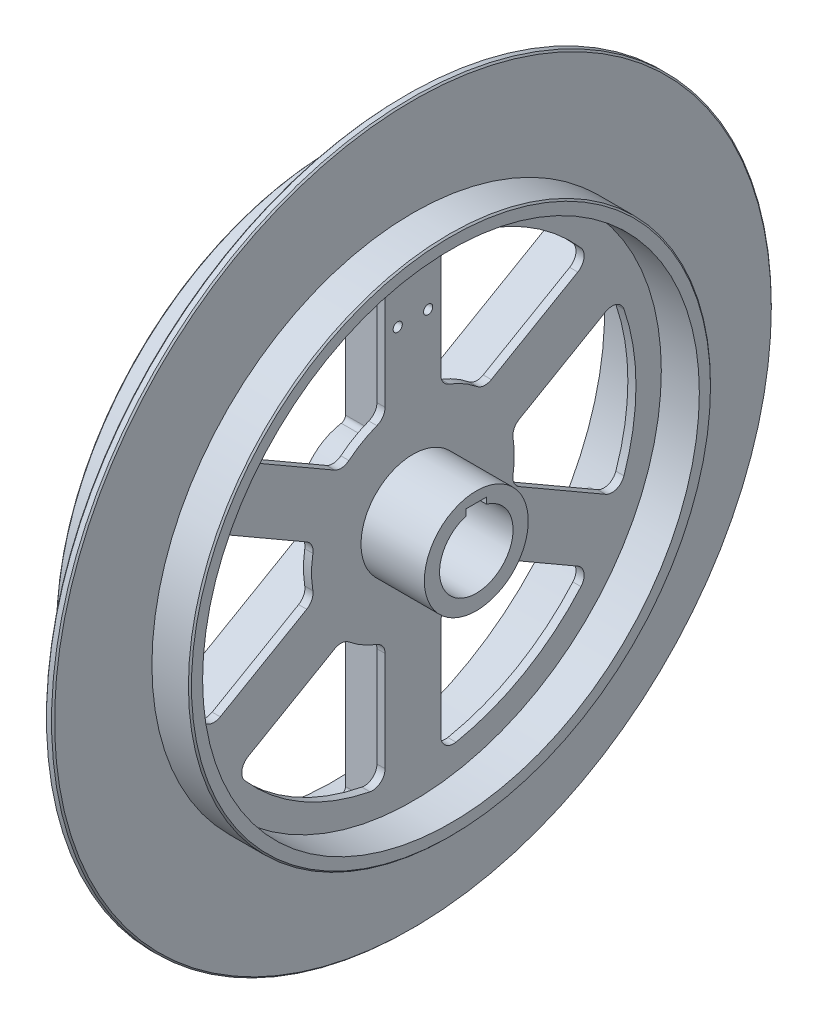
from build123d import *

# Parameters (mm, degrees)
CUT_EXTRUDE1_DEPTH       = 1014.9432923
CIRPATTERN1_COUNT        = 6
BOSS_EXTRUDE1_REACH      = 1015.943
FILLET2_R                = 10
CIRPATTERN2_COUNT        = 6
FILLET2_OF_CIRPATTERN2_R = 10
SKETCH5_R                = 9
CUT_EXTRUDE2_DEPTH       = 1014.9432923
CUT_EXTRUDE3_DEPTH       = 20
CUT_EXTRUDE3_DEPTH_BACK  = 1041.251892572
CHAMFER1_SIZE            = 3
SKETCH7_W                = 40
SKETCH7_H                = 18.8
CUT_EXTRUDE4_DEPTH       = 1035.746345729


with BuildPart() as part:
    # Sketch1 → Revolve1 (revolve)
    with BuildSketch(Plane.XY, mode=Mode.PRIVATE) as revolve1_sk:
        Polygon((0, 102.5), (79, 102.5), (79, 137.5), (109, 137.5), (109, 534), (-31, 534), (-31, 550), (109, 550), (109, 710), (125, 710), (125, 515), (200, 515), (200, 490), (125, 490), (125, 102.5), (250, 102.5), (250, 72.5), (0, 72.5), align=None)
    revolve(revolve1_sk.sketch.rotate(Axis((-373.351674541, 0, 0), (1, 0, 0)), 90), axis=Axis((-373.351674541, 0, 0), (1, 0, 0)))

    # Sketch3 → Cut-Extrude1 (cut, through all)
    with BuildSketch(Plane.ZY.offset(-109)):
        with BuildLine():
            Line((-55, 407.216158815), (-55, 210.297408448))
            ThreePointArc((-55, 210.297408448), (-59.418184941, 196.106253143), (-71.111111111, 186.931029732))
            ThreePointArc((-71.111111111, 186.931029732), (-100, 173.205080757), (-126.331464948, 155.049543579))
            ThreePointArc((-126.331464948, 155.049543579), (-140.123904592, 149.510784178), (-154.622898066, 152.780101432))
            Line((-154.622898066, 152.780101432), (-325.159538365, 251.239476616))
            ThreePointArc((-325.159538365, 251.239476616), (-337.320790629, 268.78857093), (-331.494450315, 289.329275066))
            ThreePointArc((-331.494450315, 289.329275066), (-220, 381.051177665), (-84.819277108, 431.747252719))
            ThreePointArc((-84.819277108, 431.747252719), (-64.117335358, 426.522659374), (-55, 407.216158815))
        make_face()
    cut_extrude1 = extrude(amount=-CUT_EXTRUDE1_DEPTH, mode=Mode.SUBTRACT)

    # CirPattern1: Cut-Extrude1 ×6 about axis
    cirpattern1_axis = Axis((0, 0, 0), (1, 0, 0))
    for i in range(1, CIRPATTERN1_COUNT):
        add(cut_extrude1.rotate(cirpattern1_axis, i * 360 / CIRPATTERN1_COUNT), mode=Mode.SUBTRACT)

    # Boss-Extrude1: up to this face of the body (flat: up to its plane)
    boss_extrude1_end = Plane(part.part.faces().sort_by_distance((0, 0, -75.399137803))[0])
    # Sketch4 → Boss-Extrude1 (add, up to the picked face)
    with BuildSketch(Plane.ZY.offset(-109), mode=Mode.PRIVATE) as boss_extrude1_sk1:
        with BuildLine():
            Line((-8, 533.940071544), (-8, 102.187327982))
            ThreePointArc((-8, 102.187327982), (0, 102.5), (8, 102.187327982))
            Line((8, 102.187327982), (8, 533.940071544))
            ThreePointArc((8, 533.940071544), (0, 534), (-8, 533.940071544))
        make_face()
    boss_extrude1_tool1 = split(extrude(boss_extrude1_sk1.sketch, amount=BOSS_EXTRUDE1_REACH, mode=Mode.PRIVATE), bisect_by=boss_extrude1_end, keep=Keep.BOTH, mode=Mode.PRIVATE)
    boss_extrude1 = boss_extrude1_tool1.solids().sort_by(Axis((109, 318.187922, 0), (-1, 0, 0)))[0]
    add(boss_extrude1)

    # Fillet2
    fillet2_edges = [part.edges().sort_by_distance(p)[0] for p in [
        (94, 137.267075441, 8),
        (39.5, 102.187327982, -8),
        (94, 137.267075441, -8),
        (109, 335.603573492, 8),
        (39.5, 102.187327982, 8),
        (54.5, 533.940071544, -8),
        (109, 335.603573492, -8),
        (54.5, 533.940071544, 8),
    ]]
    fillet(fillet2_edges, radius=FILLET2_R)

    # CirPattern2: Boss-Extrude1 ×6 about axis
    cirpattern2_axis = Axis((0, 0, 0), (1, 0, 0))
    for i in range(1, CIRPATTERN2_COUNT):
        add(boss_extrude1.rotate(cirpattern2_axis, i * 360 / CIRPATTERN2_COUNT))

    # Fillet2 of CirPattern2
    fillet2_of_cirpattern2_edges = [part.edges().sort_by_distance(p)[0] for p in [
        (94, 61.70533449, 122.876774435),
        (39.5, 58.021867221, 84.496821977),
        (94, 75.561740951, 114.876774435),
        (109, 160.873583516, 294.641220245),
        (39.5, 44.16546076, 92.496821977),
        (54.5, 273.898239002, 458.405666055),
        (109, 174.729989976, 286.641220245),
        (54.5, 260.041832542, 466.405666055),
        (94, -75.561740951, 114.876774435),
        (39.5, -44.16546076, 92.496821977),
        (94, -61.70533449, 122.876774435),
        (109, -174.729989976, 286.641220245),
        (39.5, -58.021867221, 84.496821977),
        (54.5, -260.041832542, 466.405666055),
        (109, -160.873583516, 294.641220245),
        (54.5, -273.898239002, 458.405666055),
        (94, -137.267075441, -8),
        (39.5, -102.187327982, 8),
        (94, -137.267075441, 8),
        (109, -335.603573492, -8),
        (39.5, -102.187327982, -8),
        (54.5, -533.940071544, 8),
        (109, -335.603573492, 8),
        (54.5, -533.940071544, -8),
        (94, -61.70533449, -122.876774435),
        (39.5, -58.021867221, -84.496821977),
        (94, -75.561740951, -114.876774435),
        (109, -160.873583516, -294.641220245),
        (39.5, -44.16546076, -92.496821977),
        (54.5, -273.898239002, -458.405666055),
        (109, -174.729989976, -286.641220245),
        (54.5, -260.041832542, -466.405666055),
        (94, 75.561740951, -114.876774435),
        (39.5, 44.16546076, -92.496821977),
        (94, 61.70533449, -122.876774435),
        (109, 174.729989976, -286.641220245),
        (39.5, 58.021867221, -84.496821977),
        (54.5, 260.041832542, -466.405666055),
        (109, 160.873583516, -294.641220245),
        (54.5, 273.898239002, -458.405666055),
    ]]
    fillet(fillet2_of_cirpattern2_edges, radius=FILLET2_OF_CIRPATTERN2_R)

    # Sketch5 → Cut-Extrude2 (cut, through all)
    with BuildSketch(Plane.ZY.offset(-109)):
        with Locations((-30, 425)):
            Circle(SKETCH5_R)
        with Locations((-30, 335)):
            Circle(SKETCH5_R)
        with Locations((30, 335)):
            Circle(SKETCH5_R)
        with Locations((30, 425)):
            Circle(SKETCH5_R)
    extrude(amount=-CUT_EXTRUDE2_DEPTH, mode=Mode.SUBTRACT)

    # Sketch6 → Cut-Extrude3 (cut, two sides: drawn at the far end of the back side and taken through both)
    with BuildSketch(Plane.XY.offset(8).offset(-CUT_EXTRUDE3_DEPTH_BACK)):
        with BuildLine():
            Line((94, 395), (109, 395))
            Line((109, 395), (109, 365))
            Line((109, 365), (94, 365))
            ThreePointArc((94, 365), (79, 380), (94, 395))
        make_face()
    extrude(amount=CUT_EXTRUDE3_DEPTH + CUT_EXTRUDE3_DEPTH_BACK, mode=Mode.SUBTRACT)

    # Chamfer1
    chamfer1_edges = [part.edges().sort_by_distance(p)[0] for p in [
        (-31, 0, -550),
        (109, 0, -710),
        (125, 0, -710),
        (200, 0, -515),
    ]]
    chamfer(chamfer1_edges, length=CHAMFER1_SIZE)

    # Sketch7 → Cut-Extrude4 (cut, through all)
    with BuildSketch(Plane.ZY):
        with Locations((0, 72.5)):
            Rectangle(SKETCH7_W, SKETCH7_H)
    extrude(amount=-CUT_EXTRUDE4_DEPTH, mode=Mode.SUBTRACT)


solid = part.part
